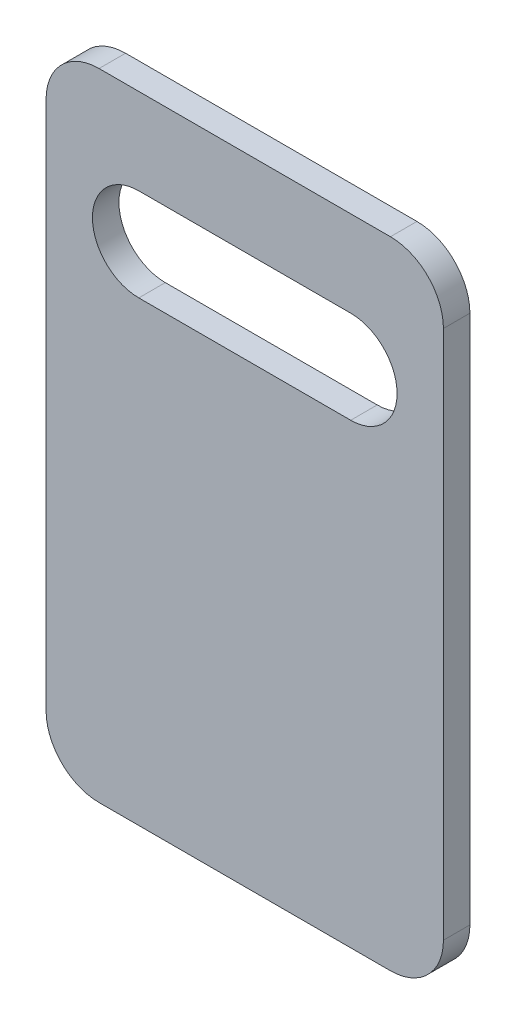
from build123d import *

# Parameters (mm, degrees)
SKETCH1_W           = 15
SKETCH1_H           = 24
BOSS_EXTRUDE1_DEPTH = 1
FILLET1_R           = 2


with BuildPart() as part:
    # Sketch1 → Boss-Extrude1 (new body)
    with BuildSketch(Plane.XY):
        Rectangle(SKETCH1_W, SKETCH1_H)
        with BuildLine():
            Line((-4, 8.75), (4, 8.75))
            ThreePointArc((4, 8.75), (5.75, 7), (4, 5.25))
            Line((4, 5.25), (-4, 5.25))
            ThreePointArc((-4, 5.25), (-5.75, 7), (-4, 8.75))
        make_face(mode=Mode.SUBTRACT)
    extrude(amount=BOSS_EXTRUDE1_DEPTH)

    # Fillet1
    fillet1_edges = [part.edges().sort_by_distance(p)[0] for p in [
        (7.5, -12, 0.5),
        (-7.5, -12, 0.5),
        (-7.5, 12, 0.5),
        (7.5, 12, 0.5),
    ]]
    fillet(fillet1_edges, radius=FILLET1_R)


solid = part.part
